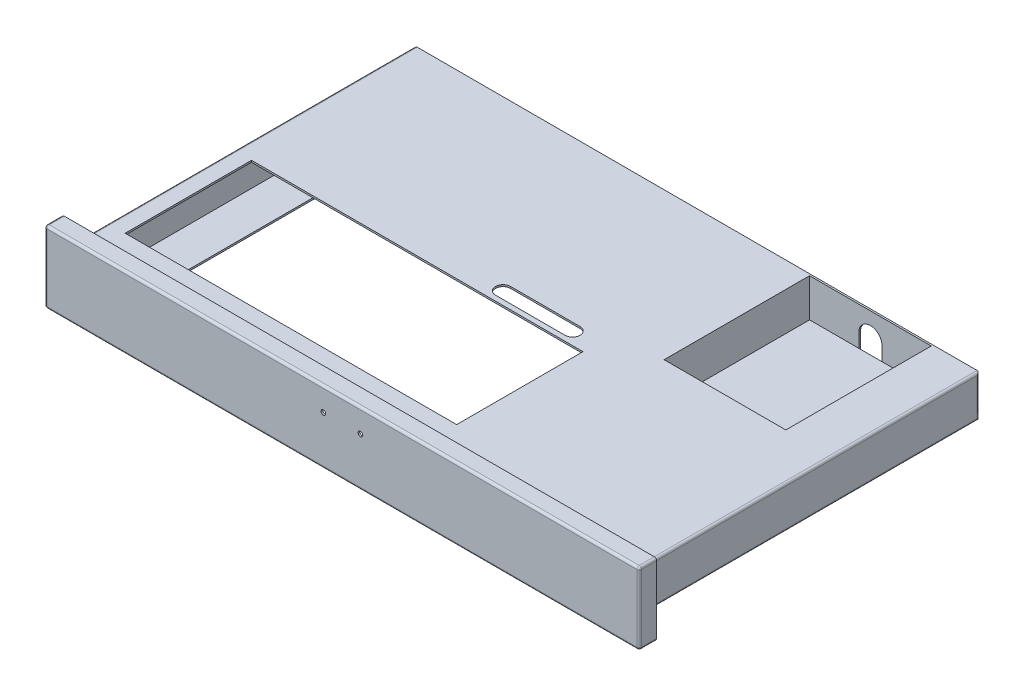
from build123d import *

# Parameters (mm, degrees)
SKETCH_1_W          = 513
SKETCH_1_H          = 62
EXTRUDE_1_DEPTH     = 15
SHELL_1_T           = 1.5
SKETCH_2_W          = 487
SKETCH_2_H          = 36
CUT_EXTRUDE_1_DEPTH = 2
EXTRUDE_2_DEPTH     = 305
SKETCH_4_W          = 484
SKETCH_4_H          = 33
EXTRUDE_3_DEPTH     = 1.5
SKETCH_6_W          = 108
SKETCH_6_H          = 127
EXTRUDE_4_DEPTH     = 33
SKETCH_7_W          = 105
SKETCH_7_H          = 125.5
CUT_EXTRUDE_2_DEPTH = 33
CUT_EXTRUDE_3_DEPTH = 1.5
SKETCH_9_W          = 286
SKETCH_9_H          = 109
CUT_EXTRUDE_4_DEPTH = 1.5
CUT_EXTRUDE_5_DEPTH = 10
SKETCH_11_R         = 2
CUT_EXTRUDE_6_DEPTH = 400.722716392
FILLET_1_R          = 2


with BuildPart() as part:
    # 草图1 → 凸台-拉伸1 (new body)
    with BuildSketch(Plane.XY):
        Rectangle(SKETCH_1_W, SKETCH_1_H)
    extrude(amount=EXTRUDE_1_DEPTH)

    # 抽壳1 (no face opened: a closed hollow body)
    add(offset(amount=-SHELL_1_T, mode=Mode.PRIVATE), mode=Mode.SUBTRACT)

    # 草图2 → 切除-拉伸1 (cut)
    with BuildSketch(Plane(origin=(0, 0, 0), x_dir=(-1, 0, 0), z_dir=(0, 0, -1))):
        Rectangle(SKETCH_2_W, SKETCH_2_H)
    extrude(amount=-CUT_EXTRUDE_1_DEPTH, mode=Mode.SUBTRACT)

    # 草图3 → 凸台-拉伸2 (add)
    with BuildSketch(Plane(origin=(0, 0, 13.5), x_dir=(-1, 0, 0), z_dir=(0, 0, -1))):
        Polygon((243.5, 18), (-243.5, 18), (-243.5, -18), (-208.5, -18), (-208.5, -16.5), (-242, -16.5), (-242, 16.5), (242, 16.5), (242, -16.5), (208.5, -16.5), (208.5, -18), (243.5, -18), align=None)
    extrude(amount=EXTRUDE_2_DEPTH)

    # 草图4 → 凸台-拉伸3 (add)
    with BuildSketch(Plane(origin=(0, 0, -291.5), x_dir=(-1, 0, 0), z_dir=(0, 0, -1))):
        Rectangle(SKETCH_4_W, SKETCH_4_H)
    extrude(amount=-EXTRUDE_3_DEPTH)

    # 草图6 → 凸台-拉伸4 (add)
    with BuildSketch(Plane.XZ.offset(-16.5)):
        with Locations((151, -226.5)):
            Rectangle(SKETCH_6_W, SKETCH_6_H)
    extrude(amount=EXTRUDE_4_DEPTH)

    # 草图7 → 切除-拉伸2 (cut)
    with BuildSketch(Plane(origin=(0, 18, 0), x_dir=(1, 0, 0), z_dir=(0, 1, 0))):
        with Locations((151, 227.25)):
            Rectangle(SKETCH_7_W, SKETCH_7_H)
    extrude(amount=-CUT_EXTRUDE_2_DEPTH, mode=Mode.SUBTRACT)

    # 草图8 → 切除-拉伸3 (cut)
    with BuildSketch(Plane(origin=(0, 0, -291.5), x_dir=(-1, 0, 0), z_dir=(0, 0, -1))):
        with BuildLine():
            Line((-161, -18), (-161, -3))
            ThreePointArc((-161, -3), (-151, 7), (-141, -3))
            Line((-141, -3), (-141, -18))
            Line((-141, -18), (-161, -18))
        make_face()
    extrude(amount=-CUT_EXTRUDE_3_DEPTH, mode=Mode.SUBTRACT)

    # 草图9 → 切除-拉伸4 (cut)
    with BuildSketch(Plane(origin=(0, 18, 0), x_dir=(1, 0, 0), z_dir=(0, 1, 0))):
        with Locations((-85.5, 81)):
            Rectangle(SKETCH_9_W, SKETCH_9_H)
    extrude(amount=-CUT_EXTRUDE_4_DEPTH, mode=Mode.SUBTRACT)

    # 草图10 → 切除-拉伸5 (cut)
    with BuildSketch(Plane(origin=(0, 18, 0), x_dir=(1, 0, 0), z_dir=(0, 1, 0))):
        with BuildLine():
            Line((-22.5, 153), (37.5, 153))
            ThreePointArc((37.5, 153), (44, 146.5), (37.5, 140))
            Line((37.5, 140), (-22.5, 140))
            ThreePointArc((-22.5, 140), (-29, 146.5), (-22.5, 153))
        make_face()
    extrude(amount=-CUT_EXTRUDE_5_DEPTH, mode=Mode.SUBTRACT)

    # 草图11 → 切除-拉伸6 (cut, through all)
    with BuildSketch(Plane(origin=(0, 0, 13.5), x_dir=(-1, 0, 0), z_dir=(0, 0, -1))):
        with Locations((-16, 11)):
            Circle(SKETCH_11_R)
        with Locations((16, 11)):
            Circle(SKETCH_11_R)
    extrude(amount=-CUT_EXTRUDE_6_DEPTH, mode=Mode.SUBTRACT)

    # 圆角1
    fillet_1_edges = [part.edges().sort_by_distance(p)[0] for p in [
        (-256.5, 0, 15),
        (0, -31, 15),
        (-243.5, 0, 0),
        (0, 18, 0),
        (243.5, 0, 0),
        (226, -18, 0),
        (256.5, 0, 15),
        (-243.5, -18, -145.75),
        (-243.5, 18, -145.75),
        (243.5, 18, -145.75),
        (243.5, -18, -145.75),
        (-226, -18, 0),
        (-243.5, 0, -291.5),
        (243.5, 0, -291.5),
        (0, 31, 15),
        (256.5, -31, 7.5),
        (-256.5, -31, 7.5),
        (-256.5, 31, 7.5),
        (256.5, 31, 7.5),
    ]]
    fillet(fillet_1_edges, radius=FILLET_1_R)


solid = part.part
